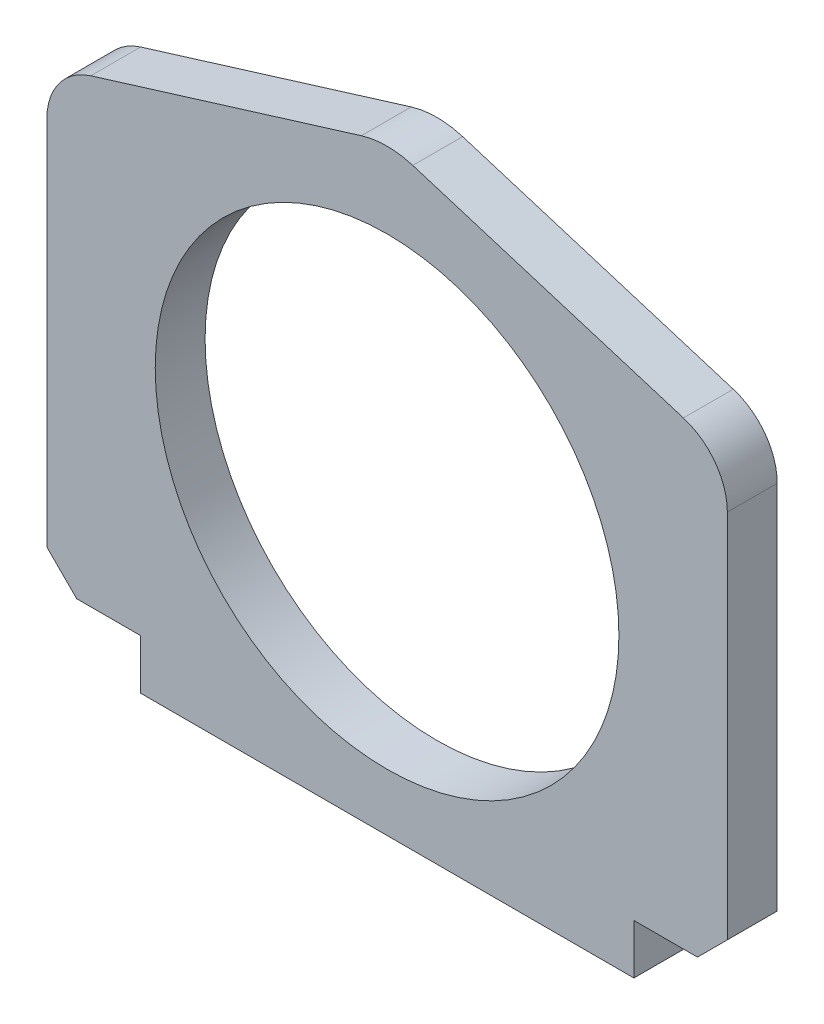
SolidWorks part; units mm, degrees
ref_plane "Front Plane" through (0, 0, 0) normal (0, 0, 1) x (1, 0, 0)
ref_plane "Top Plane" through (0, 0, 0) normal (0, 1, 0) x (1, 0, 0)
ref_plane "Right Plane" through (0, 0, 0) normal (1, 0, 0) x (0, 0, -1)
sketch "Sketch1" plane through (0, 0, 0) normal (0, 0, 1) x (1, 0, 0)
  line L0 (-99, 0) -> (99, 0)
  line L1 (99, 0) -> (99, 20)
  line L2 (99, 20) -> (124.5, 20)
  line L3 (136.5, 32) -> (136.5, 180.6)
  line L4 (0, 0) -> (0, 341.4194) construction
  line L5 (124.5, 20) -> (136.5, 32)
  line L6 (10.3085, 237.9475) -> (118.8632, 204.4911)
  line L7 (-124.5, 20) -> (-136.5, 32)
  line L8 (-99, 20) -> (-124.5, 20)
  line L9 (-99, 0) -> (-99, 20)
  line L10 (-136.5, 32) -> (-136.5, 180.6)
  line L11 (-10.3085, 237.9475) -> (-118.8632, 204.4911)
  arc A0 (10.3085, 237.9475) -> (-10.3085, 237.9475) centre (0, 204.5) ccw
  arc A1 (136.5, 180.6) -> (118.8632, 204.4911) centre (111.5, 180.6) ccw
  arc A2 (-136.5, 180.6) -> (-118.8632, 204.4911) centre (-111.5, 180.6) cw
  circle A3 centre (0, 116) radius 93
  point P5 (136.5, 20)
  point P18 (-136.5, 20)
  dimension "D1" = 70
  dimension "D6" = 50
  dimension "D9" = 186
  dimension "D2" = 204.5
  dimension "D3" = 198
  dimension "D4" = 273
  dimension "D5" = 20
  dimension "D7" = 160.6
  dimension "D10" = 96
extrude "Boss-Extrude1" add sketch "Sketch1" along normal blind 20
